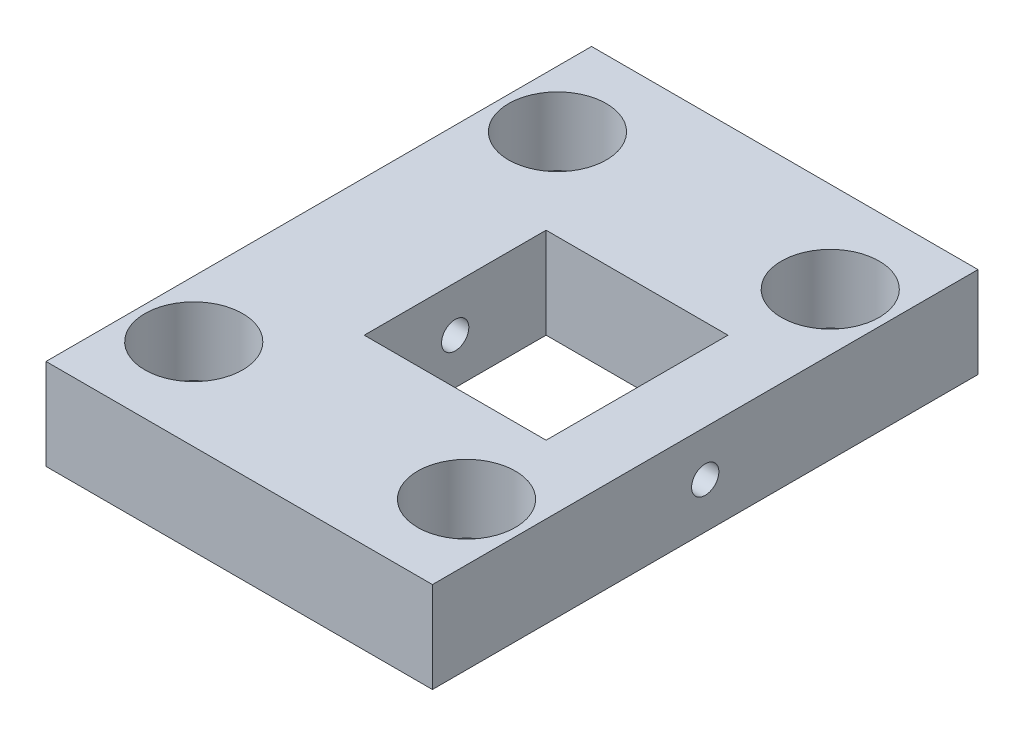
from build123d import *

# Parameters (mm, degrees)
SKETCH1_W           = 85
SKETCH1_H           = 120
SKETCH1_R           = 5.5
SKETCH1_W_2         = 40
SKETCH1_H_2         = 40
BOSS_EXTRUDE1_DEPTH = 20
SKETCH2_R           = 10.75
CUT_EXTRUDE1_DEPTH  = 15
SKETCH3_R           = 3
CUT_EXTRUDE2_DEPTH  = 106.948100502


with BuildPart() as part:
    # Sketch1 → Boss-Extrude1 (new body)
    with BuildSketch(Plane(origin=(0, 0, 0), x_dir=(1, 0, 0), z_dir=(0, 1, 0))):
        Rectangle(SKETCH1_W, SKETCH1_H)
        with Locations(Location((-30, 40, 0), (0, 0, 270))):
            Circle(SKETCH1_R, mode=Mode.SUBTRACT)
        with Locations(Location((30, 40, 0), (0, 0, 270))):
            Circle(SKETCH1_R, mode=Mode.SUBTRACT)
        with Locations(Location((30, -40, 0), (0, 0, 270))):
            Circle(SKETCH1_R, mode=Mode.SUBTRACT)
        with Locations(Location((-30, -40, 0), (0, 0, 270))):
            Circle(SKETCH1_R, mode=Mode.SUBTRACT)
        with Locations((7.5, 0)):
            Rectangle(SKETCH1_W_2, SKETCH1_H_2, mode=Mode.SUBTRACT)
    extrude(amount=BOSS_EXTRUDE1_DEPTH)

    # Sketch2 → Cut-Extrude1 (cut)
    with BuildSketch(Plane(origin=(0, 20, 0), x_dir=(1, 0, 0), z_dir=(0, 1, 0))):
        with Locations(Location((30, 40, 0), (0, 0, 270))):
            Circle(SKETCH2_R)
        with Locations(Location((-30, 40, 0), (0, 0, 270))):
            Circle(SKETCH2_R)
        with Locations(Location((-30, -40, 0), (0, 0, 270))):
            Circle(SKETCH2_R)
        with Locations(Location((30, -40, 0), (0, 0, 270))):
            Circle(SKETCH2_R)
    extrude(amount=-CUT_EXTRUDE1_DEPTH, mode=Mode.SUBTRACT)

    # Sketch3 → Cut-Extrude2 (cut, through all)
    with BuildSketch(Plane.ZY.offset(42.5)):
        with Locations((0, 10)):
            Circle(SKETCH3_R)
    extrude(amount=-CUT_EXTRUDE2_DEPTH, mode=Mode.SUBTRACT)


solid = part.part
